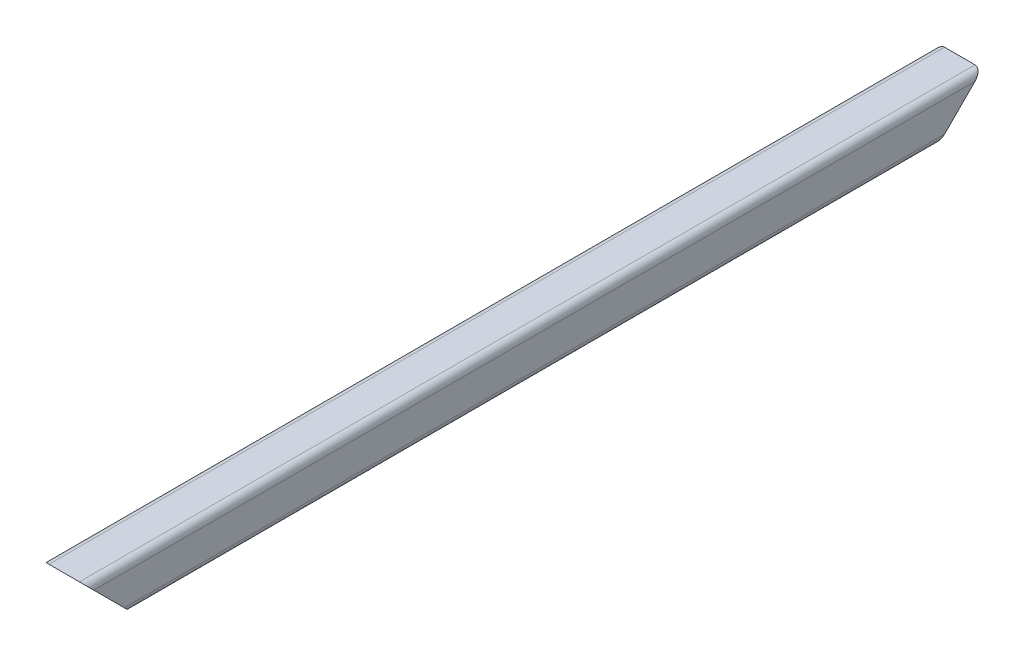
SolidWorks part; units mm, degrees
material "AISI 1045 钢，冷拔"
ref_plane "Front Plane" through (0, 0, 0) normal (0, 0, 1) x (1, 0, 0)
ref_plane "Top Plane" through (0, 0, 0) normal (0, 1, 0) x (1, 0, 0)
ref_plane "Right Plane" through (0, 0, 0) normal (1, 0, 0) x (0, 0, -1)
sketch "Sketch1" plane through (0, 0, 0) normal (0, 0, 1) x (1, 0, 0)
  line L0 (-21.0947, 0) -> (28.2454, 0) construction
  line L1 (0, 28.305) -> (0, -28.2454) construction
  line L2 (-17, 21) -> (17, 21)
  line L3 (-17, -25) -> (17, -25)
  line L4 (-25, -17) -> (-25, 17)
  line L5 (-17, 25) -> (17, 25)
  line L6 (25, -17) -> (25, 17)
  line L7 (-25, -25) -> (25, 25) construction
  line L8 (-25, 25) -> (25, -25) construction
  line L9 (21, -17) -> (21, 17)
  line L10 (-17, -21) -> (17, -21)
  line L11 (-21, -17) -> (-21, 17)
  arc A0 (17, -25) -> (25, -17) centre (17, -17) ccw
  arc A1 (-17, -25) -> (-25, -17) centre (-17, -17) cw
  arc A2 (17, 25) -> (25, 17) centre (17, 17) cw
  arc A3 (-25, 17) -> (-17, 25) centre (-17, 17) cw
  arc A4 (-21, 17) -> (-17, 21) centre (-17, 17) cw
  arc A5 (17, 21) -> (21, 17) centre (17, 17) cw
  arc A6 (17, -21) -> (21, -17) centre (17, -17) ccw
  arc A7 (-17, -21) -> (-21, -17) centre (-17, -17) cw
  point P5 (0, 0)
  dimension "D3" = 8
  dimension "D1" = 50
  dimension "D2" = 50
  dimension "D4" = 4
extrude "Boss-Extrude1" add sketch "Sketch1" along normal mid plane 1000
sketch "Sketch2" plane through (-25, 0, 0) normal (-1, 0, 0) x (0, 0, 1)
  line L0 (-500, 25) -> (-450, -25)
  line L1 (500, -25) -> (-500, -25) construction
  line L2 (-450, -25) -> (-500, -25)
  line L3 (-500, -25) -> (-500, 25)
  dimension "D1" = 45
extrude "Cut-Extrude1" cut sketch "Sketch2" against normal through all
mirror "Mirror1" about plane through (0, 0, 0) normal (0, 0, 1) of "Cut-Extrude1"
